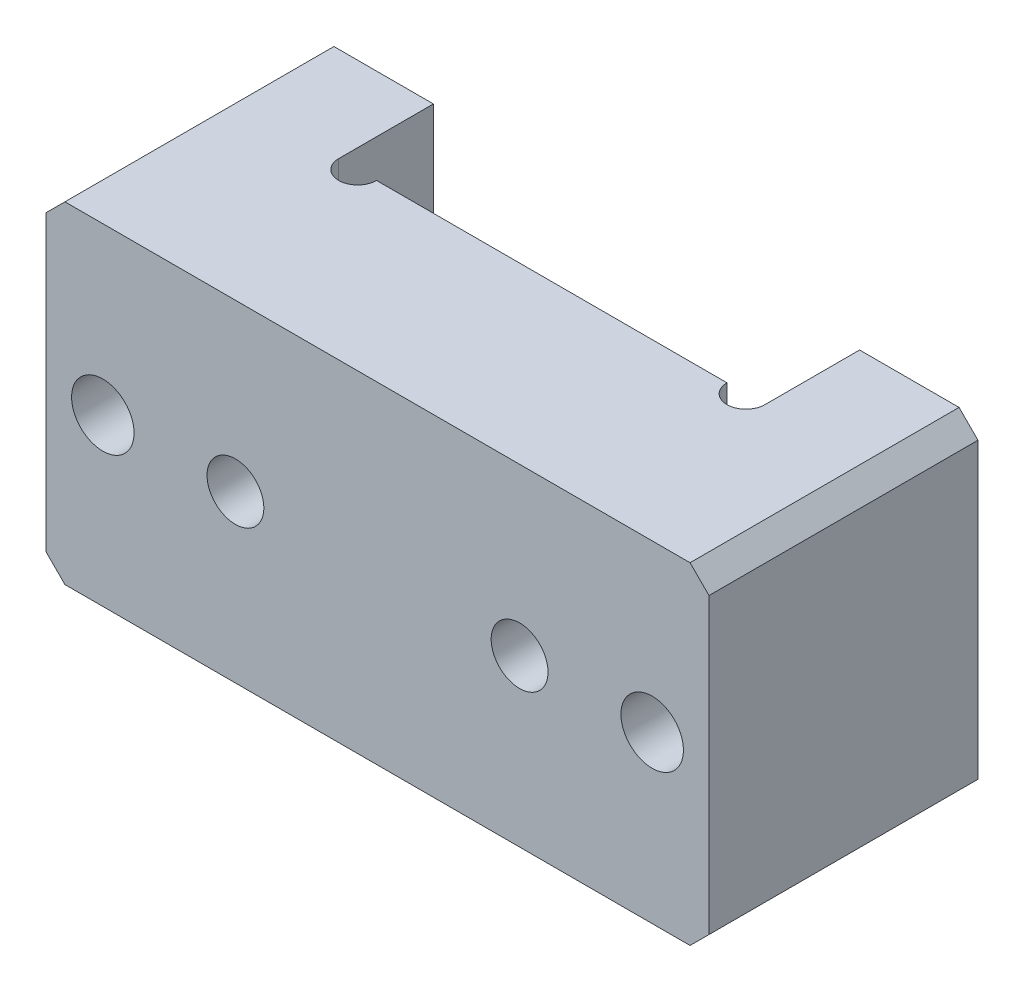
from build123d import *

# Parameters (mm, degrees)
EXTRUDE_1_DEPTH              = 17.5
CUT_EXTRUDE_1_REACH          = 59.066
SKETCH_2_R                   = 2
CHAMFER_1_SIZE               = 2
F_6_0MM_1_D                  = 6
F_6_0MM_1_DEPTH              = 15
F_6_0MM_1_TIP                = 1.802581857
HOLE_WIZARD_M6_1_D           = 6.6
HOLE_WIZARD_M6_1_CBORE_D     = 11
HOLE_WIZARD_M6_1_CBORE_DEPTH = 6.8
HOLE_WIZARD_M4_1_D           = 3.3
HOLE_WIZARD_M4_1_DEPTH       = 18.5
HOLE_WIZARD_M4_1_TIP         = 0.991420021


with BuildPart() as part:
    # 草图1 → 凸台-拉伸1 (new, symmetric)
    with BuildSketch(Plane(origin=(0, 0, 0), x_dir=(1, 0, 0), z_dir=(0, 1, 0))):
        Polygon((-35, 0), (35, 0), (35, 28.4), (22.5, 28.4), (22.5, 18.4), (-22.5, 18.4), (-22.5, 28.4), (-35, 28.4), align=None)
    extrude(amount=EXTRUDE_1_DEPTH, both=True)

    # 草图2 → 切除-拉伸1 (cut, up to next)
    with BuildSketch(Plane(origin=(0, 17.5, 0), x_dir=(1, 0, 0), z_dir=(0, 1, 0)), mode=Mode.PRIVATE) as cut_extrude_1_sk1:
        with Locations((20.5, 18.4)):
            Circle(SKETCH_2_R)
    cut_extrude_1_tool1 = extrude(cut_extrude_1_sk1.sketch, amount=-CUT_EXTRUDE_1_REACH, mode=Mode.PRIVATE) & part.part
    # 草图2 → 切除-拉伸1 (cut, up to next)
    with BuildSketch(Plane(origin=(0, 17.5, 0), x_dir=(1, 0, 0), z_dir=(0, 1, 0)), mode=Mode.PRIVATE) as cut_extrude_1_sk2:
        with Locations((-20.5, 18.4)):
            Circle(SKETCH_2_R)
    cut_extrude_1_tool2 = extrude(cut_extrude_1_sk2.sketch, amount=-CUT_EXTRUDE_1_REACH, mode=Mode.PRIVATE) & part.part
    add(cut_extrude_1_tool1.solids().sort_by_distance((20.5, 17.5, -18.4))[0], mode=Mode.SUBTRACT)
    add(cut_extrude_1_tool2.solids().sort_by_distance((-20.5, 17.5, -18.4))[0], mode=Mode.SUBTRACT)

    # 倒角1
    chamfer_1_edges = [part.edges().sort_by_distance(p)[0] for p in [
        (35, -17.5, -14.2),
        (-35, -17.5, -14.2),
        (35, 17.5, -14.2),
        (-35, 17.5, -14.2),
    ]]
    chamfer(chamfer_1_edges, length=CHAMFER_1_SIZE)

    # Ø6.0mm 暗销孔1
    with Locations(Plane.XY):
        with Locations((-15, 0), (15, 0)):
            Hole(F_6_0MM_1_D / 2, depth=F_6_0MM_1_DEPTH)
            with Locations((0, 0, -(F_6_0MM_1_DEPTH + F_6_0MM_1_TIP / 2))):  # 118° drill point
                Cone(0, F_6_0MM_1_D / 2, F_6_0MM_1_TIP, mode=Mode.SUBTRACT)

    # M6 六角圆柱头螺钉的柱形沉头孔1 (through all)
    with Locations(Plane(origin=(0, 0, -28.4), x_dir=(-1, 0, 0), z_dir=(0, 0, -1))):
        with Locations((-29, 0), (29, 0)):
            CounterBoreHole(HOLE_WIZARD_M6_1_D / 2, HOLE_WIZARD_M6_1_CBORE_D / 2, HOLE_WIZARD_M6_1_CBORE_DEPTH)

    # M4 螺纹孔1
    with Locations(Plane(origin=(0, 0, -28.4), x_dir=(-1, 0, 0), z_dir=(0, 0, -1))):
        with Locations((-29, 12.5), (-29, -12.5), (29, 12.5), (29, -12.5)):
            Hole(HOLE_WIZARD_M4_1_D / 2, depth=HOLE_WIZARD_M4_1_DEPTH)
            with Locations((0, 0, -(HOLE_WIZARD_M4_1_DEPTH + HOLE_WIZARD_M4_1_TIP / 2))):  # 118° drill point
                Cone(0, HOLE_WIZARD_M4_1_D / 2, HOLE_WIZARD_M4_1_TIP, mode=Mode.SUBTRACT)


solid = part.part
